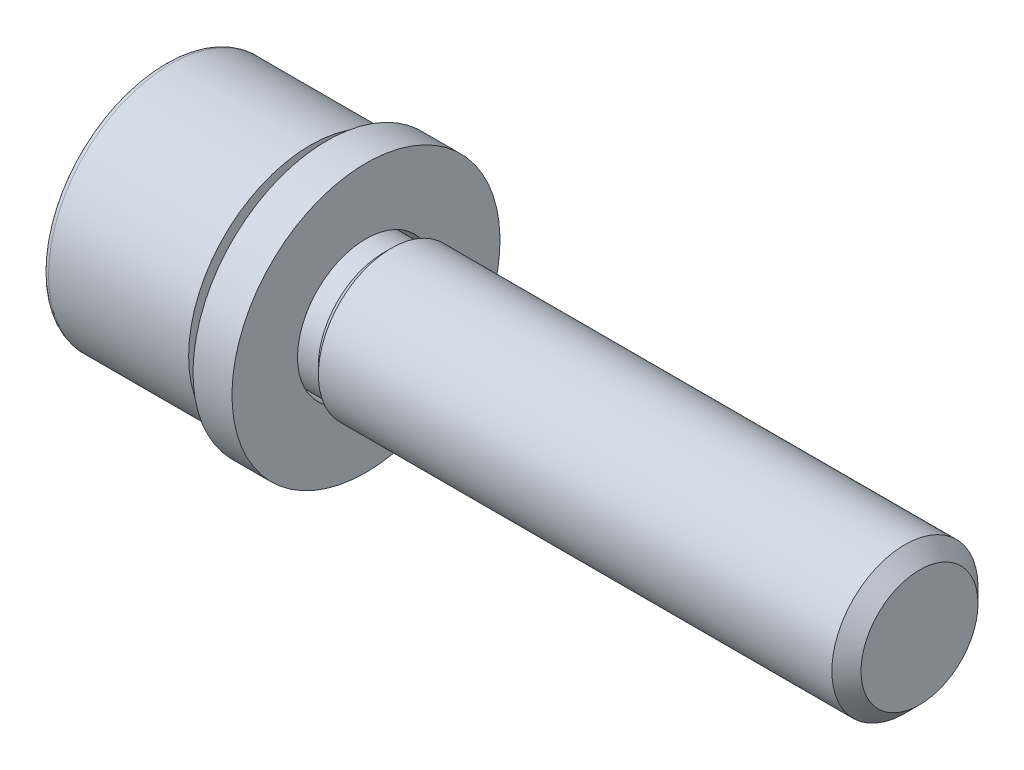
SolidWorks part; units mm, degrees
ref_plane "Front Plane" through (0, 0, 0) normal (0, 0, 1) x (1, 0, 0)
ref_plane "Top Plane" through (0, 0, 0) normal (0, 1, 0) x (1, 0, 0)
ref_plane "Right Plane" through (0, 0, 0) normal (1, 0, 0) x (0, 0, -1)
sketch "Dimension Sketch" plane through (0, 0, 0) normal (0, 0, 1) x (1, 0, 0)
  line L0 (0, 0) -> (31, 0) construction
  point P2 (6.8, 0)
  point P3 (25.28, 0)
  point P4 (30, 0)
  point P5 (3, 0)
  point P6 (10, 0)
  point P7 (6, 0)
  point P8 (6, 0)
  point P9 (15.35, 0)
  point P10 (16.03, 0)
  point P11 (0.25, 0)
  point P12 (7, 0)
  point P14 (20.28, 0)
  point P15 (16.63, 0)
  point P16 (0, 9.38)
  point P17 (0, 7.08)
  dimension "k" = 6
  dimension "l" = 25
  dimension "t" = 3
  dimension "dk" = 10
  dimension "d" = 6
  dimension "da" = 6.8
  dimension "b" = 24
  dimension "e" = 5.72
  dimension "p" = 1
  dimension "ds" = 5.35
  dimension "lf" = 0.68
  dimension "r" = 0.25
  dimension "s" = 5
  dimension "v" = 0.6
  dimension "dw" = 9.38
  dimension "w" = 2.3
sketch "Sketch1" plane through (0, 0, 0) normal (0, 0, 1) x (1, 0, 0)
  line L1 (0, 0) -> (0, 5)
  line L2 (0, 5) -> (6, 5)
  line L3 (6, 5) -> (6, 3.4)
  line L4 (6.68, 2.675) -> (9, 2.675)
  line L5 (31, 3) -> (31, 0)
  line L6 (0, 0) -> (31, 0)
  line L7 (0, 0) -> (-33.993, 0) construction
  line L8 (6.0647, 3.2322) -> (6.4947, 2.7572)
  line L9 (9, 2.675) -> (9.325, 3)
  line L10 (9.325, 3) -> (31, 3)
  line L11 (5.3512, 0) -> (3.7, 2.86) construction
  line L12 (3.7, 2.86) -> (0, 2.86) construction
  line L13 (5.3512, 0) -> (3.7, -2.86) construction
  line L14 (3.7, -2.86) -> (0, -2.86) construction
  arc A0 (6.68, 2.675) -> (6.4947, 2.7572) centre (6.68, 2.925) cw
  arc A1 (6.0647, 3.2322) -> (6, 3.4) centre (6.25, 3.4) cw
  point P10 (3.7, 5)
  point P21 (0.634, 5)
  dimension "D1" = 0.25
  dimension "D2" = 6
  dimension "dk" = 10
  dimension "D3" = 6
  dimension "l" = 25
  dimension "D5" = 45
  dimension "da" = 6.8
  dimension "lt" = 0.68
  dimension "ds" = 5.35
  dimension "ls" = 3
  dimension "D6" = 120
  dimension "w" = 2.3
  dimension "D7" = 5.72
  dimension "f" = 0.634
revolve "Base-Revolve" add sketch "Sketch1" angle 360 about L7
cosmetic thread "Cosmetic Thread1" parameters "D1"=22, "D2"=4.9175
sketch "Sketch2" plane through (0, 0, 0) normal (-1, 0, 0) x (0, 0, 1)
  line L1 (2.4768, -1.43) -> (2.4768, 1.43)
  line L2 (2.4768, 1.43) -> (0, 2.86)
  line L3 (0, 2.86) -> (-2.4768, 1.43)
  line L4 (-2.4768, 1.43) -> (-2.4768, -1.43)
  line L5 (-2.4768, -1.43) -> (0, -2.86)
  line L6 (0, -2.86) -> (2.4768, -1.43)
  circle A0 centre (0, 0) radius 2.4768 construction
  dimension "e" = 5.72
extrude "Cut-Extrude1" cut sketch "Sketch2" against normal up to vertex (3.7 mm away) up to point (3.7, 2.86, 0)
ref_plane "Plane1" through (5.3512, 0, 0) normal (1, 0, 0) x (0, 0, -1)
sketch "Sketch13" plane through (0, 0, 0) normal (0, 0, 1) x (1, 0, 0)
  line L0 (0, 2.86) -> (0.3832, 2.4768)
  line L1 (0.3832, 2.4768) -> (0, 2.4768)
  line L2 (0, 0) -> (0, 5) construction
  line L3 (0, 2.4768) -> (0, 2.86)
  line L6 (0, 0) -> (-33.993, 0) construction
  line L7 (0, 0) -> (-33.993, 0) construction
  line L8 (3.7, 2.86) -> (0, 2.86) construction
  line L9 (3.7, 2.86) -> (0, 2.86) construction
  line L10 (1.85, 2.86) -> (1.85, 0) construction
  line L11 (0, 0) -> (31, 0) construction
  line L12 (3.7, 2.4768) -> (3.7, 2.86) construction
  line L13 (3.3168, 2.4768) -> (3.7, 2.4768) construction
  line L14 (3.7, 2.86) -> (3.3168, 2.4768) construction
  dimension "D1" = 45
revolve "Cut-Revolve4" cut sketch "Sketch13" angle 360 mid plane about L7
sketch "Sketch16" plane through (0, 0, 0) normal (0, 0, 1) x (1, 0, 0)
  line L0 (5.3512, 0) -> (3.7, 2.86) construction
  line L1 (0, 0) -> (31, 0) construction
  line L2 (5.3512, 0) -> (3.7, 2.86)
  line L3 (3.7, 0) -> (5.3512, 0)
  line L4 (3.7, 2.86) -> (3.7, 0)
revolve "Cut-Revolve5" cut sketch "Sketch16" angle 360 mid plane about L3
fillet "Fillet1" radius 0.25 1 edges at (0, 0, -5)
sketch "Sketch11" plane through (0, 0, 0) normal (0, 0, 1) x (1, 0, 0)
  line L0 (6.68, 2.81) -> (6.68, 5.5)
  line L1 (6.68, 5.5) -> (8.28, 5.5)
  line L2 (8.28, 5.5) -> (8.28, 2.81)
  line L3 (8.28, 2.81) -> (6.68, 2.81)
  line L4 (0, 0) -> (31, 0) construction
  line L5 (0, 0) -> (31, 0) construction
  dimension "垫圈d" = 5.62
  dimension "h" = 1.6
  dimension "d2" = 11
revolve "Revolve1" add sketch "Sketch11" angle 360 mid plane about L5
chamfer "Chamfer1" distance 0.6 angle 45 1 edges at (31, 0, -3)
